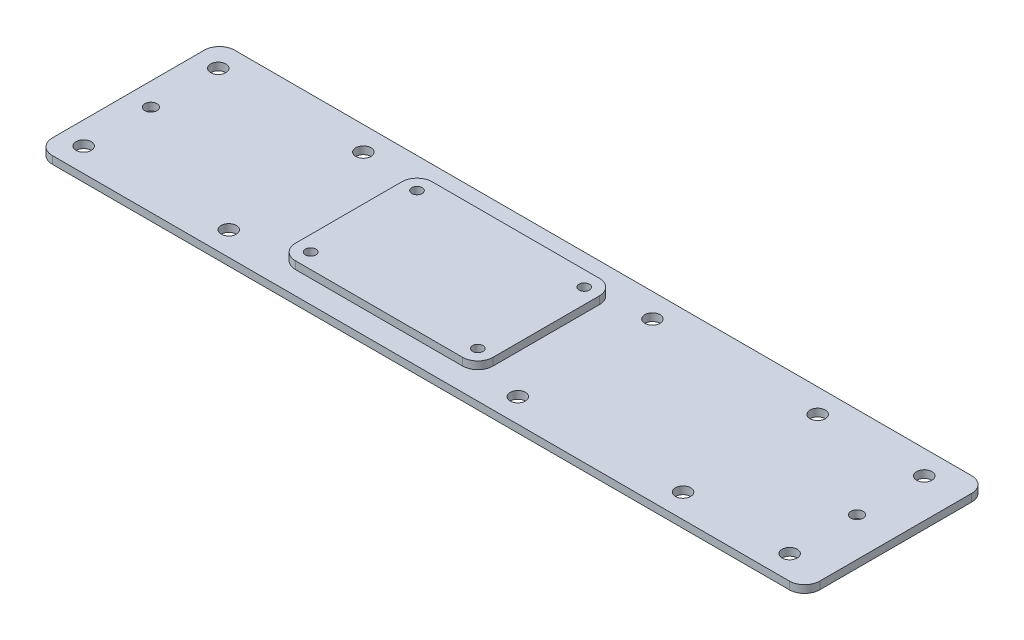
from build123d import *

# Parameters (mm, degrees)
SKETCH1_W                  = 505
SKETCH1_H                  = 120
SKETCH1_W_2                = 100
SKETCH1_H_2                = 60
BOSS_EXTRUDE1_DEPTH        = 5
FILLET1_R                  = 10
FILLET2_R                  = 10
BOSS_EXTRUDE2_DEPTH        = 5
M8_TAPPED_HOLE1_AT_2_COUNT = 2
M8_TAPPED_HOLE1_AT_2_PITCH = 110
M8_TAPPED_HOLE1_AT_3_COUNT = 2
M8_TAPPED_HOLE1_AT_3_PITCH = 70
M8_TAPPED_HOLE1_AT_4_COUNT = 2
M8_TAPPED_HOLE1_AT_4_PITCH = 130.384048104
SKETCH5_R                  = 5
SKETCH5_R_2                = 4
CUT_EXTRUDE1_DEPTH         = 20


with BuildPart() as part:
    # Sketch1 → Boss-Extrude1 (new body)
    with BuildSketch(Plane(origin=(0, 539, 0), x_dir=(1, 0, 0), z_dir=(0, 1, 0))):
        with Locations((42.5, 129.05)):
            Rectangle(SKETCH1_W, SKETCH1_H)
        with Locations((0, 129.05)):
            Rectangle(SKETCH1_W_2, SKETCH1_H_2, mode=Mode.SUBTRACT)
    extrude(amount=BOSS_EXTRUDE1_DEPTH)

    # Fillet1
    fillet1_edges = [part.edges().sort_by_distance(p)[0] for p in [
        (-210, 541.5, -189.05),
        (295, 541.5, -189.05),
        (295, 541.5, -69.05),
        (-210, 541.5, -69.05),
    ]]
    fillet(fillet1_edges, radius=FILLET1_R)

    # Fillet2
    fillet2_edges = [part.edges().sort_by_distance(p)[0] for p in [
        (-50, 541.5, -159.05),
        (-50, 541.5, -99.05),
        (50, 541.5, -99.05),
        (50, 541.5, -159.05),
    ]]
    fillet(fillet2_edges, radius=FILLET2_R)


with BuildPart() as body_2:
    # Sketch2 → Boss-Extrude2 (new body)
    with BuildSketch(Plane(origin=(0, 544, 0), x_dir=(1, 0, 0), z_dir=(0, 1, 0))):
        with BuildLine():
            Line((-55, 174.05), (55, 174.05))
            ThreePointArc((55, 174.05), (62.071067812, 171.121067812), (65, 164.05))
            Line((65, 164.05), (65, 94.05))
            ThreePointArc((65, 94.05), (62.071067812, 86.978932188), (55, 84.05))
            Line((55, 84.05), (-55, 84.05))
            ThreePointArc((-55, 84.05), (-62.071067812, 86.978932188), (-65, 94.05))
            Line((-65, 94.05), (-65, 164.05))
            ThreePointArc((-65, 164.05), (-62.071067812, 171.121067812), (-55, 174.05))
        make_face()
    extrude(amount=BOSS_EXTRUDE2_DEPTH)


with BuildPart() as m8_tapped_hole1_tool:
    # Sketch4 → M8 Tapped Hole1 (revolve)
    with BuildSketch(Plane(origin=(-55, 549, -164.05), x_dir=(0, 0, 1), z_dir=(1, 0, 0))):
        Polygon((0, 0), (0, 22.25), (3.4, 20.207073895), (3.4, 0), align=None)
    m8_tapped_hole1 = revolve(axis=Axis((-55, 555.35, -164.05), (0, -1, 0)))


with BuildPart() as part_1:
    add(part.part)

    # M8 Tapped Hole1: cut by m8_tapped_hole1_tool
    add(m8_tapped_hole1_tool.part, mode=Mode.SUBTRACT)


with BuildPart() as body_2_1:
    add(body_2.part)

    # M8 Tapped Hole1: cut by m8_tapped_hole1_tool
    add(m8_tapped_hole1_tool.part, mode=Mode.SUBTRACT)


with BuildPart() as m8_tapped_hole1_at_2_tool:
    # M8 Tapped Hole1 at 2: M8 Tapped Hole1 ×2
    with Locations(*[(i * M8_TAPPED_HOLE1_AT_2_PITCH, 0, 0) for i in range(1, M8_TAPPED_HOLE1_AT_2_COUNT)]):
        add(m8_tapped_hole1)


with BuildPart() as part_2:
    add(part_1.part)

    # M8 Tapped Hole1 at 2: cut by m8_tapped_hole1_at_2_tool
    add(m8_tapped_hole1_at_2_tool.part, mode=Mode.SUBTRACT)


with BuildPart() as body_2_2:
    add(body_2_1.part)

    # M8 Tapped Hole1 at 2: cut by m8_tapped_hole1_at_2_tool
    add(m8_tapped_hole1_at_2_tool.part, mode=Mode.SUBTRACT)


with BuildPart() as m8_tapped_hole1_at_3_tool:
    # M8 Tapped Hole1 at 3: M8 Tapped Hole1 ×2
    with Locations(*[(0, 0, i * M8_TAPPED_HOLE1_AT_3_PITCH) for i in range(1, M8_TAPPED_HOLE1_AT_3_COUNT)]):
        add(m8_tapped_hole1)


with BuildPart() as part_3:
    add(part_2.part)

    # M8 Tapped Hole1 at 3: cut by m8_tapped_hole1_at_3_tool
    add(m8_tapped_hole1_at_3_tool.part, mode=Mode.SUBTRACT)


with BuildPart() as body_2_3:
    add(body_2_2.part)

    # M8 Tapped Hole1 at 3: cut by m8_tapped_hole1_at_3_tool
    add(m8_tapped_hole1_at_3_tool.part, mode=Mode.SUBTRACT)


with BuildPart() as m8_tapped_hole1_at_4_tool:
    # M8 Tapped Hole1 at 4: M8 Tapped Hole1 ×2
    with Locations(*[Vector(0.8436614877321076, 0, 0.5368754921931594) * (i * M8_TAPPED_HOLE1_AT_4_PITCH) for i in range(1, M8_TAPPED_HOLE1_AT_4_COUNT)]):
        add(m8_tapped_hole1)


with BuildPart() as part_4:
    add(part_3.part)

    # M8 Tapped Hole1 at 4: cut by m8_tapped_hole1_at_4_tool
    add(m8_tapped_hole1_at_4_tool.part, mode=Mode.SUBTRACT)

    # Sketch5 → Cut-Extrude1 (cut)
    with BuildSketch(Plane(origin=(0, 544, 0), x_dir=(1, 0, 0), z_dir=(0, 1, 0))):
        with Locations(Location((-195.060881063, 173.331788152, 0), (0, 0, 270))):
            Circle(SKETCH5_R)
        with Locations(Location((-99.578535876, 173.331788152, 0), (0, 0, 270))):
            Circle(SKETCH5_R)
        with Locations(Location((90.625449249, 173.331788152, 0), (0, 0, 270))):
            Circle(SKETCH5_R)
        with Locations(Location((199.333046544, 173.331788152, 0), (0, 0, 270))):
            Circle(SKETCH5_R)
        with Locations(Location((269.476624658, 173.331788152, 0), (0, 0, 270))):
            Circle(SKETCH5_R)
        with Locations(Location((269.476624658, 129.05, 0), (0, 0, 270))):
            Circle(SKETCH5_R_2)
        with Locations(Location((-195.060881063, 129.05, 0), (0, 0, 270))):
            Circle(SKETCH5_R_2)
        with Locations(Location((269.476624658, 84.768211848, 0), (0, 0, 90))):
            Circle(SKETCH5_R)
        with Locations(Location((199.333046544, 84.768211848, 0), (0, 0, 90))):
            Circle(SKETCH5_R)
        with Locations(Location((90.625449249, 84.768211848, 0), (0, 0, 90))):
            Circle(SKETCH5_R)
        with Locations(Location((-99.578535876, 84.768211848, 0), (0, 0, 90))):
            Circle(SKETCH5_R)
        with Locations(Location((-195.060881063, 84.768211848, 0), (0, 0, 90))):
            Circle(SKETCH5_R)
    extrude(amount=-CUT_EXTRUDE1_DEPTH, mode=Mode.SUBTRACT)


with BuildPart() as body_2_4:
    add(body_2_3.part)

    # M8 Tapped Hole1 at 4: cut by m8_tapped_hole1_at_4_tool
    add(m8_tapped_hole1_at_4_tool.part, mode=Mode.SUBTRACT)


solid = Compound([part_4.part, body_2_4.part])
